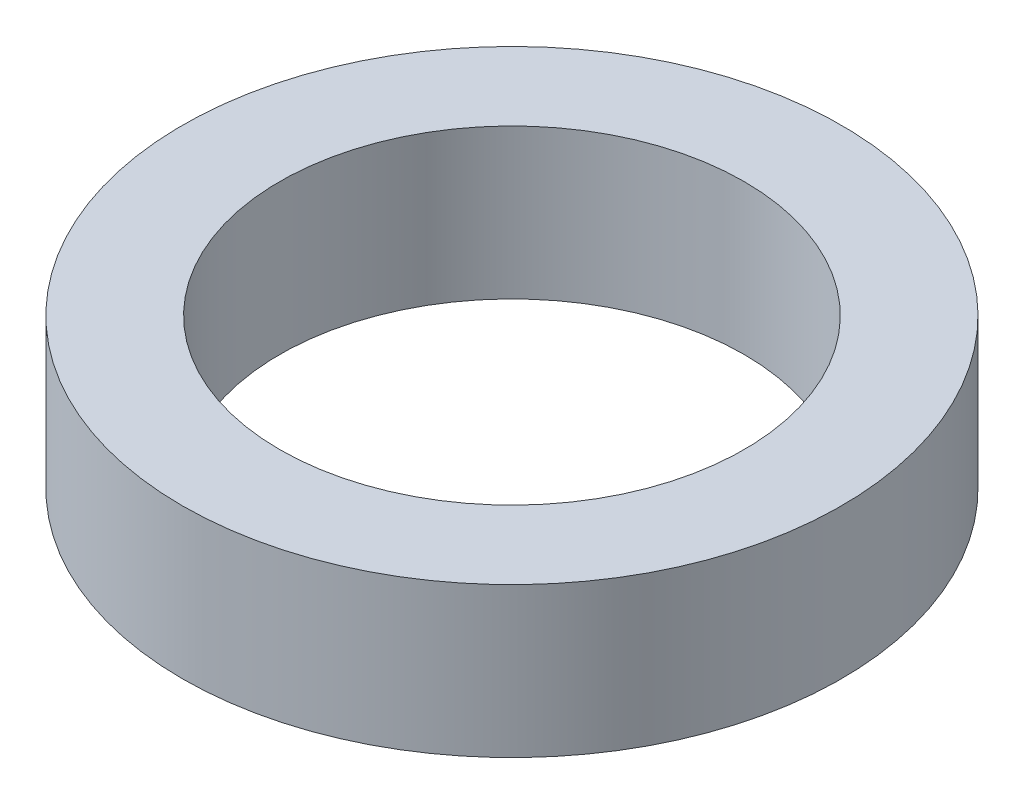
from build123d import *

# Parameters (mm, degrees)
SKETCH2_R           = 11
BOSS_EXTRUDE1_DEPTH = 5
M18_TAPPED_HOLE1_D  = 15.5


with BuildPart() as part:
    # Sketch2 → Boss-Extrude1 (new body)
    with BuildSketch(Plane(origin=(0, 0, 0), x_dir=(1, 0, 0), z_dir=(0, 1, 0))):
        with Locations(Location((0, 0, 0), (0, 0, 270))):
            Circle(SKETCH2_R)
    extrude(amount=BOSS_EXTRUDE1_DEPTH)

    # M18 Tapped Hole1 (through all)
    with Locations(Plane(origin=(0, 5, 0), x_dir=(1, 0, 0), z_dir=(0, 1, 0))):
        with Locations((0, 0)):
            Hole(M18_TAPPED_HOLE1_D / 2)


solid = part.part
